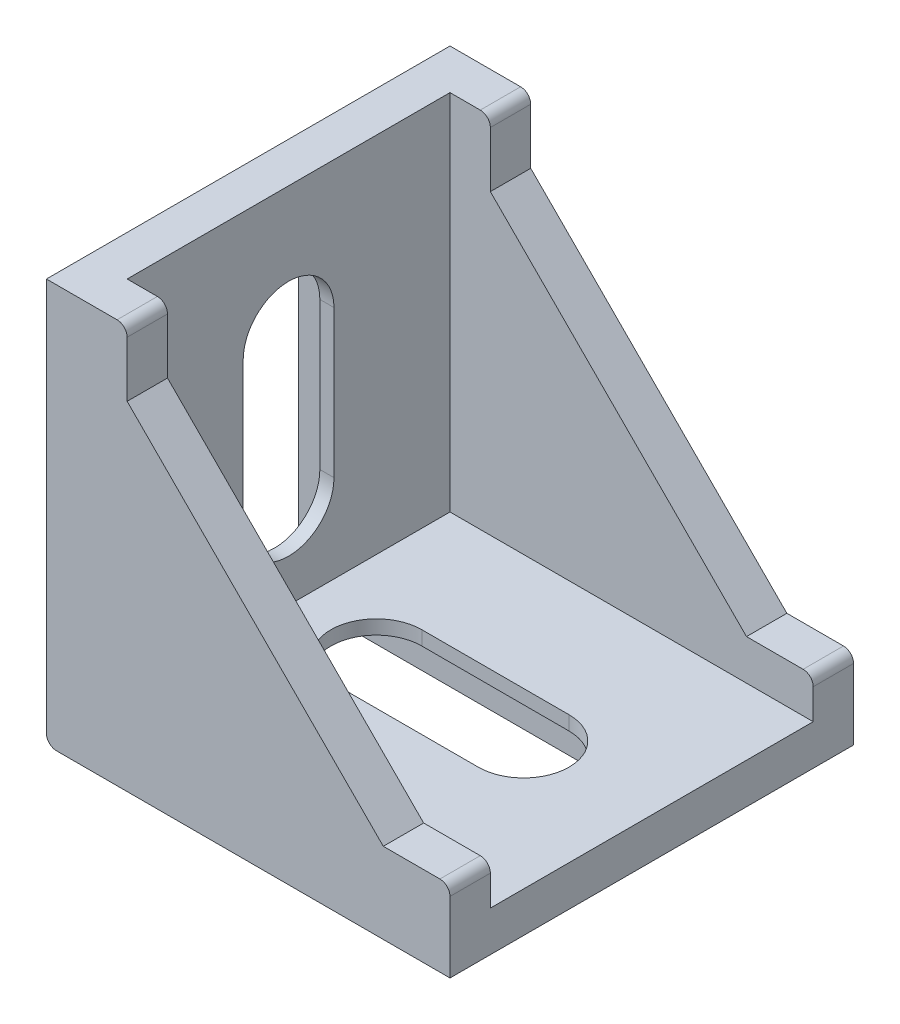
from build123d import *

# Parameters (mm, degrees)
SKETCH1_W            = 40
SKETCH1_H            = 40
BOSS_EXTRUDE1_DEPTH  = 40
CUT_EXTRUDE1_DEPTH   = 40
SKETCH3_W            = 36
SKETCH3_H            = 32
CUT_EXTRUDE2_DEPTH   = 36
SKETCH4_W            = 36
SKETCH4_H            = 6
SKETCH4_W_2          = 29
SKETCH4_H_2          = 10
CUT_EXTRUDE3_DEPTH   = 2.6
BOSS_EXTRUDE2_DEPTH  = 10
SKETCH6_W            = 35.3
SKETCH6_H            = 1.25
CUT_EXTRUDE4_DEPTH   = 10
BOSS_EXTRUDE3_DEPTH  = 6
LPATTERN1_COUNT      = 2
LPATTERN1_PITCH      = 28.4
CUT_EXTRUDE5_DEPTH   = 5
MIRROR1_COPY_1_DEPTH = 6
FILLET1_R            = 1


with BuildPart() as part:
    # Sketch1 → Boss-Extrude1 (new body)
    with BuildSketch(Plane.XY):
        with Locations((-20, 20)):
            Rectangle(SKETCH1_W, SKETCH1_H)
    extrude(amount=BOSS_EXTRUDE1_DEPTH)

    # Sketch2 → Cut-Extrude1 (cut)
    with BuildSketch(Plane.XY.offset(40)):
        Polygon((-32, 40), (-32, 33.5), (-6.610595609, 8), (0, 8), (17.085067255, 36.265731876), (-7.495565519, 45.713912599), align=None)
    extrude(amount=-CUT_EXTRUDE1_DEPTH, mode=Mode.SUBTRACT)

    # Sketch3 → Cut-Extrude2 (cut)
    with BuildSketch(Plane(origin=(0, 40, 0), x_dir=(1, 0, 0), z_dir=(0, 1, 0))):
        with Locations((-18, -20)):
            Rectangle(SKETCH3_W, SKETCH3_H)
    extrude(amount=-CUT_EXTRUDE2_DEPTH, mode=Mode.SUBTRACT)

    # Sketch4 → Cut-Extrude3 (cut)
    with BuildSketch(Plane.XZ):
        with Locations((-19.8, 34.2)):
            Rectangle(SKETCH4_W, SKETCH4_H)
        with Locations((-20.5, 20)):
            Rectangle(SKETCH4_W_2, SKETCH4_H_2)
        with Locations((-19.8, 5.8)):
            Rectangle(SKETCH4_W, SKETCH4_H)
    cut_extrude3 = extrude(amount=-CUT_EXTRUDE3_DEPTH, mode=Mode.SUBTRACT)

    # Sketch5 → Boss-Extrude2 (add)
    with BuildSketch(Plane(origin=(0, 0, 25), x_dir=(-1, 0, 0), z_dir=(0, 0, -1))):
        Polygon((31.8, 2.6), (35, 2.6), (38, 2.6), (38, -2.5), align=None)
        Polygon((6, 0), (6, -2.5), (2.7, 0), align=None)
    boss_extrude2 = extrude(amount=BOSS_EXTRUDE2_DEPTH)

    # Sketch6 → Cut-Extrude4 (cut)
    with BuildSketch(Plane.XZ):
        with Locations((-20.35, 15.625)):
            Rectangle(SKETCH6_W, SKETCH6_H)
        with Locations((-20.35, 24.375)):
            Rectangle(SKETCH6_W, SKETCH6_H)
    cut_extrude4 = extrude(amount=CUT_EXTRUDE4_DEPTH, mode=Mode.SUBTRACT)

    # Sketch7 → Boss-Extrude3 (add)
    with BuildSketch(Plane(origin=(0, 0, 8.8), x_dir=(-1, 0, 0), z_dir=(0, 0, -1))):
        Polygon((37.8, 0), (34.3, 2.6), (37.8, 2.6), align=None)
    boss_extrude3 = extrude(amount=BOSS_EXTRUDE3_DEPTH)

    # LPattern1: Boss-Extrude3 ×2
    with Locations(*[(0, 0, i * LPATTERN1_PITCH) for i in range(1, LPATTERN1_COUNT)]):
        add(boss_extrude3)

    # Sketch9 → Cut-Extrude5 (cut)
    with BuildSketch(Plane.XZ.offset(-2.6)):
        with BuildLine():
            Line((-27.3, 24.5), (-12.7, 24.5))
            ThreePointArc((-12.7, 24.5), (-8.2, 20), (-12.7, 15.5))
            Line((-12.7, 15.5), (-27.3, 15.5))
            ThreePointArc((-27.3, 15.5), (-31.8, 20), (-27.3, 24.5))
        make_face()
    cut_extrude5 = extrude(amount=-CUT_EXTRUDE5_DEPTH, mode=Mode.SUBTRACT)

    # Mirror1: Cut-Extrude3, Boss-Extrude2, Cut-Extrude4, Boss-Extrude3, Cut-Extrude5 across plane
    add(cut_extrude3.mirror(Plane(origin=(-20, 20, 0), x_dir=(0, 0, 1), z_dir=(-0.7071067811865475, 0.7071067811865477, 0))), mode=Mode.SUBTRACT)
    add(boss_extrude2.mirror(Plane(origin=(-20, 20, 0), x_dir=(0, 0, 1), z_dir=(-0.7071067811865475, 0.7071067811865477, 0))))
    add(cut_extrude4.mirror(Plane(origin=(-20, 20, 0), x_dir=(0, 0, 1), z_dir=(-0.7071067811865475, 0.7071067811865477, 0))), mode=Mode.SUBTRACT)
    add(boss_extrude3.mirror(Plane(origin=(-20, 20, 0), x_dir=(0, 0, 1), z_dir=(-0.7071067811865475, 0.7071067811865477, 0))))
    add(cut_extrude5.mirror(Plane(origin=(-20, 20, 0), x_dir=(0, 0, 1), z_dir=(-0.7071067811865475, 0.7071067811865477, 0))), mode=Mode.SUBTRACT)

    # Mirror1 copy 1 sketch → Mirror1 copy 1 (add)
    with BuildSketch(Plane(origin=(-40, 40, 37.2), x_dir=(0, -1, 0), z_dir=(0, 0, -1))):
        Polygon((37.8, 0), (34.3, -2.6), (37.8, -2.6), align=None)
    extrude(amount=MIRROR1_COPY_1_DEPTH)

    # Fillet1
    fillet1_edges = [part.edges().sort_by_distance(p)[0] for p in [
        (-32, 40, 2),
        (0, 8, 2),
        (-32, 40, 38),
        (0, 8, 38),
        (-40, 0, 20),
    ]]
    fillet(fillet1_edges, radius=FILLET1_R)


solid = part.part
